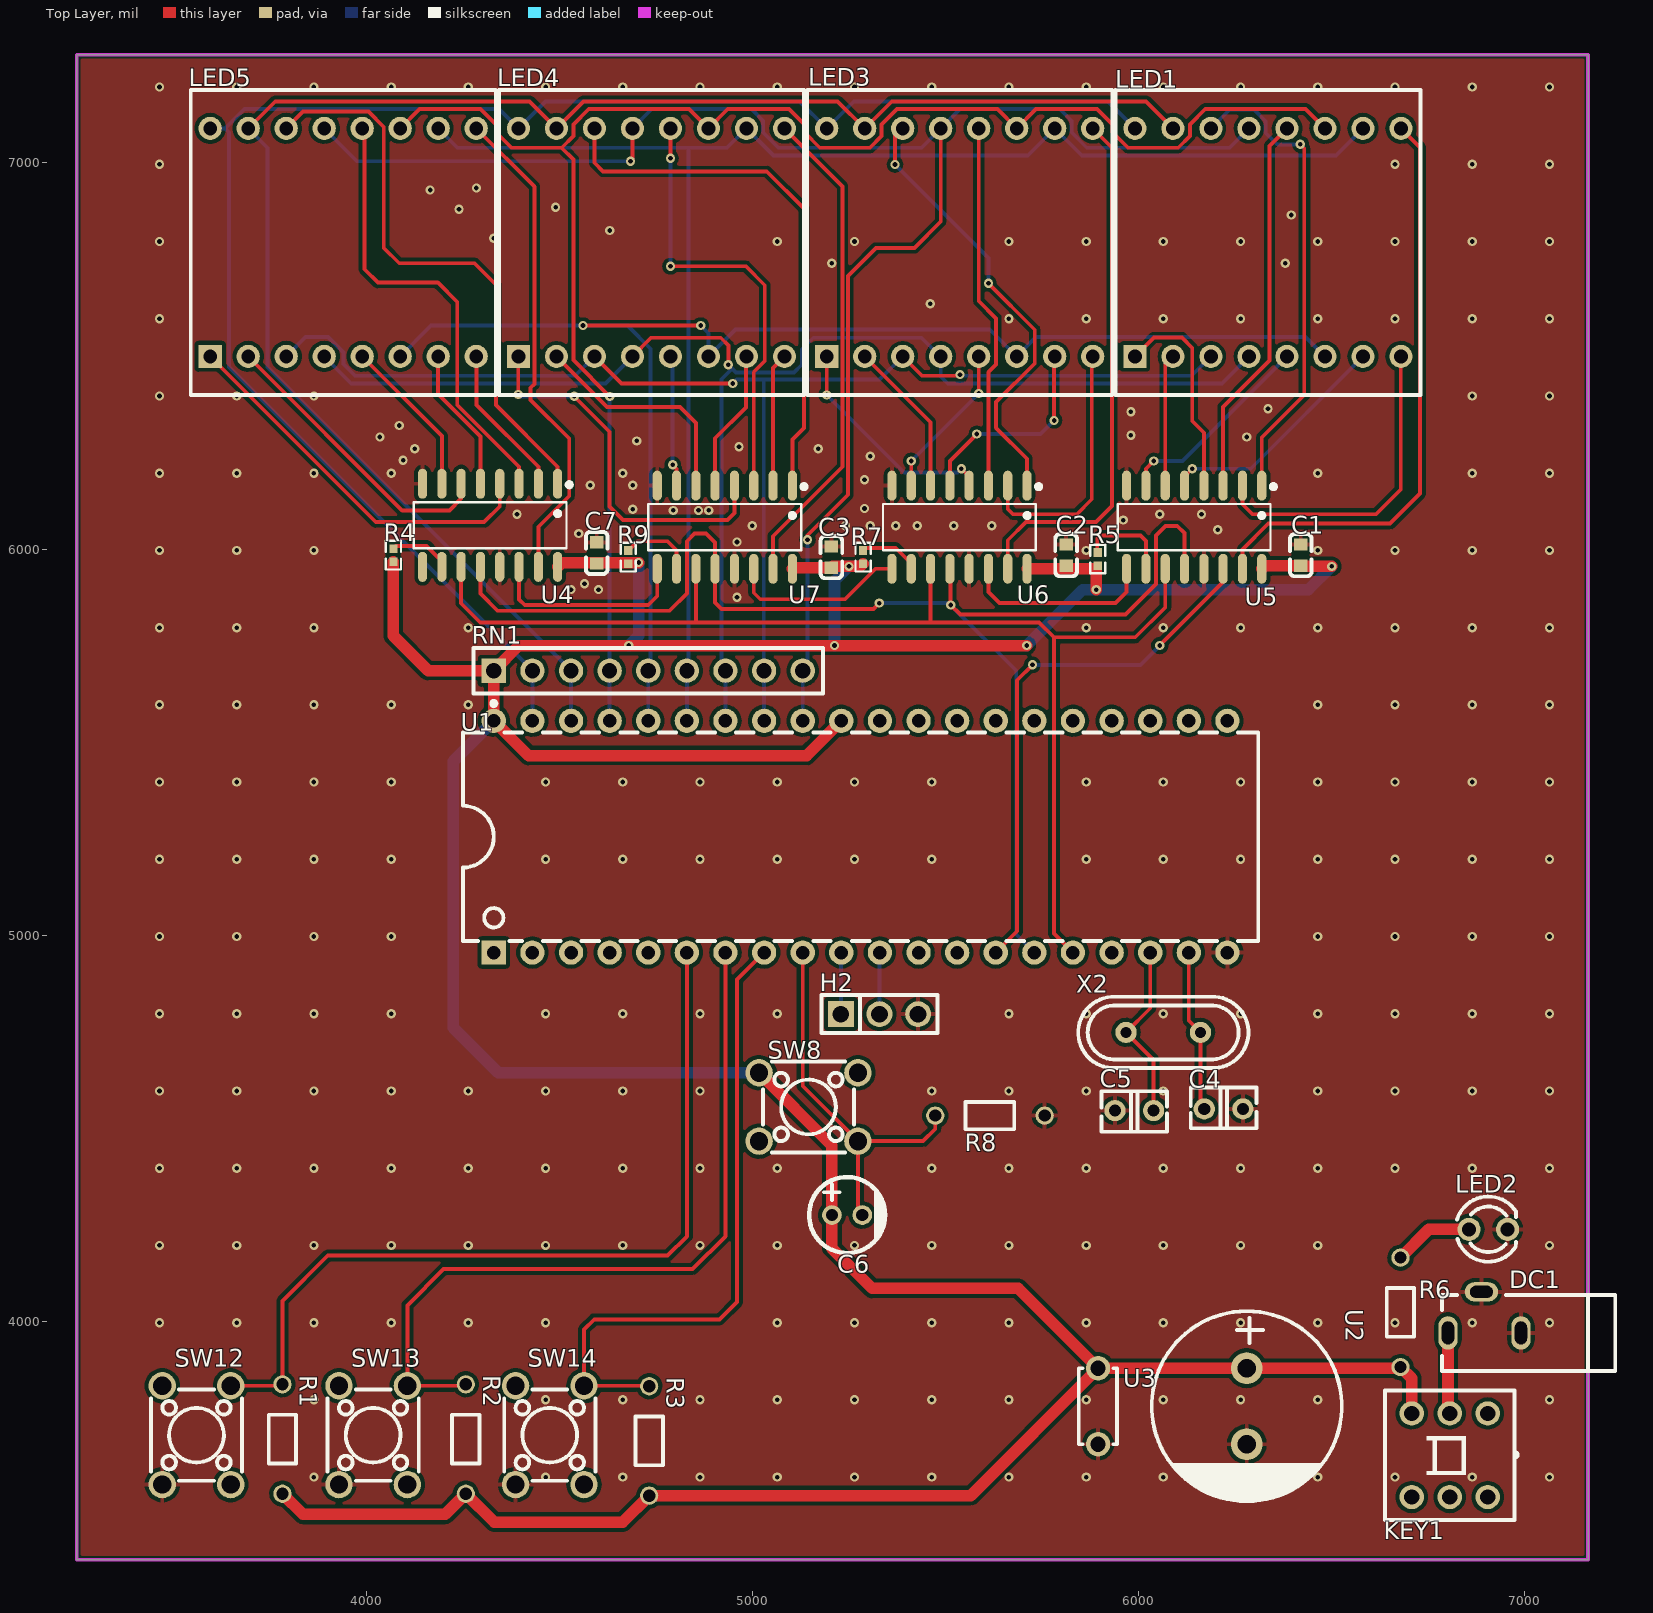
[diagram p0: Top Layer view]
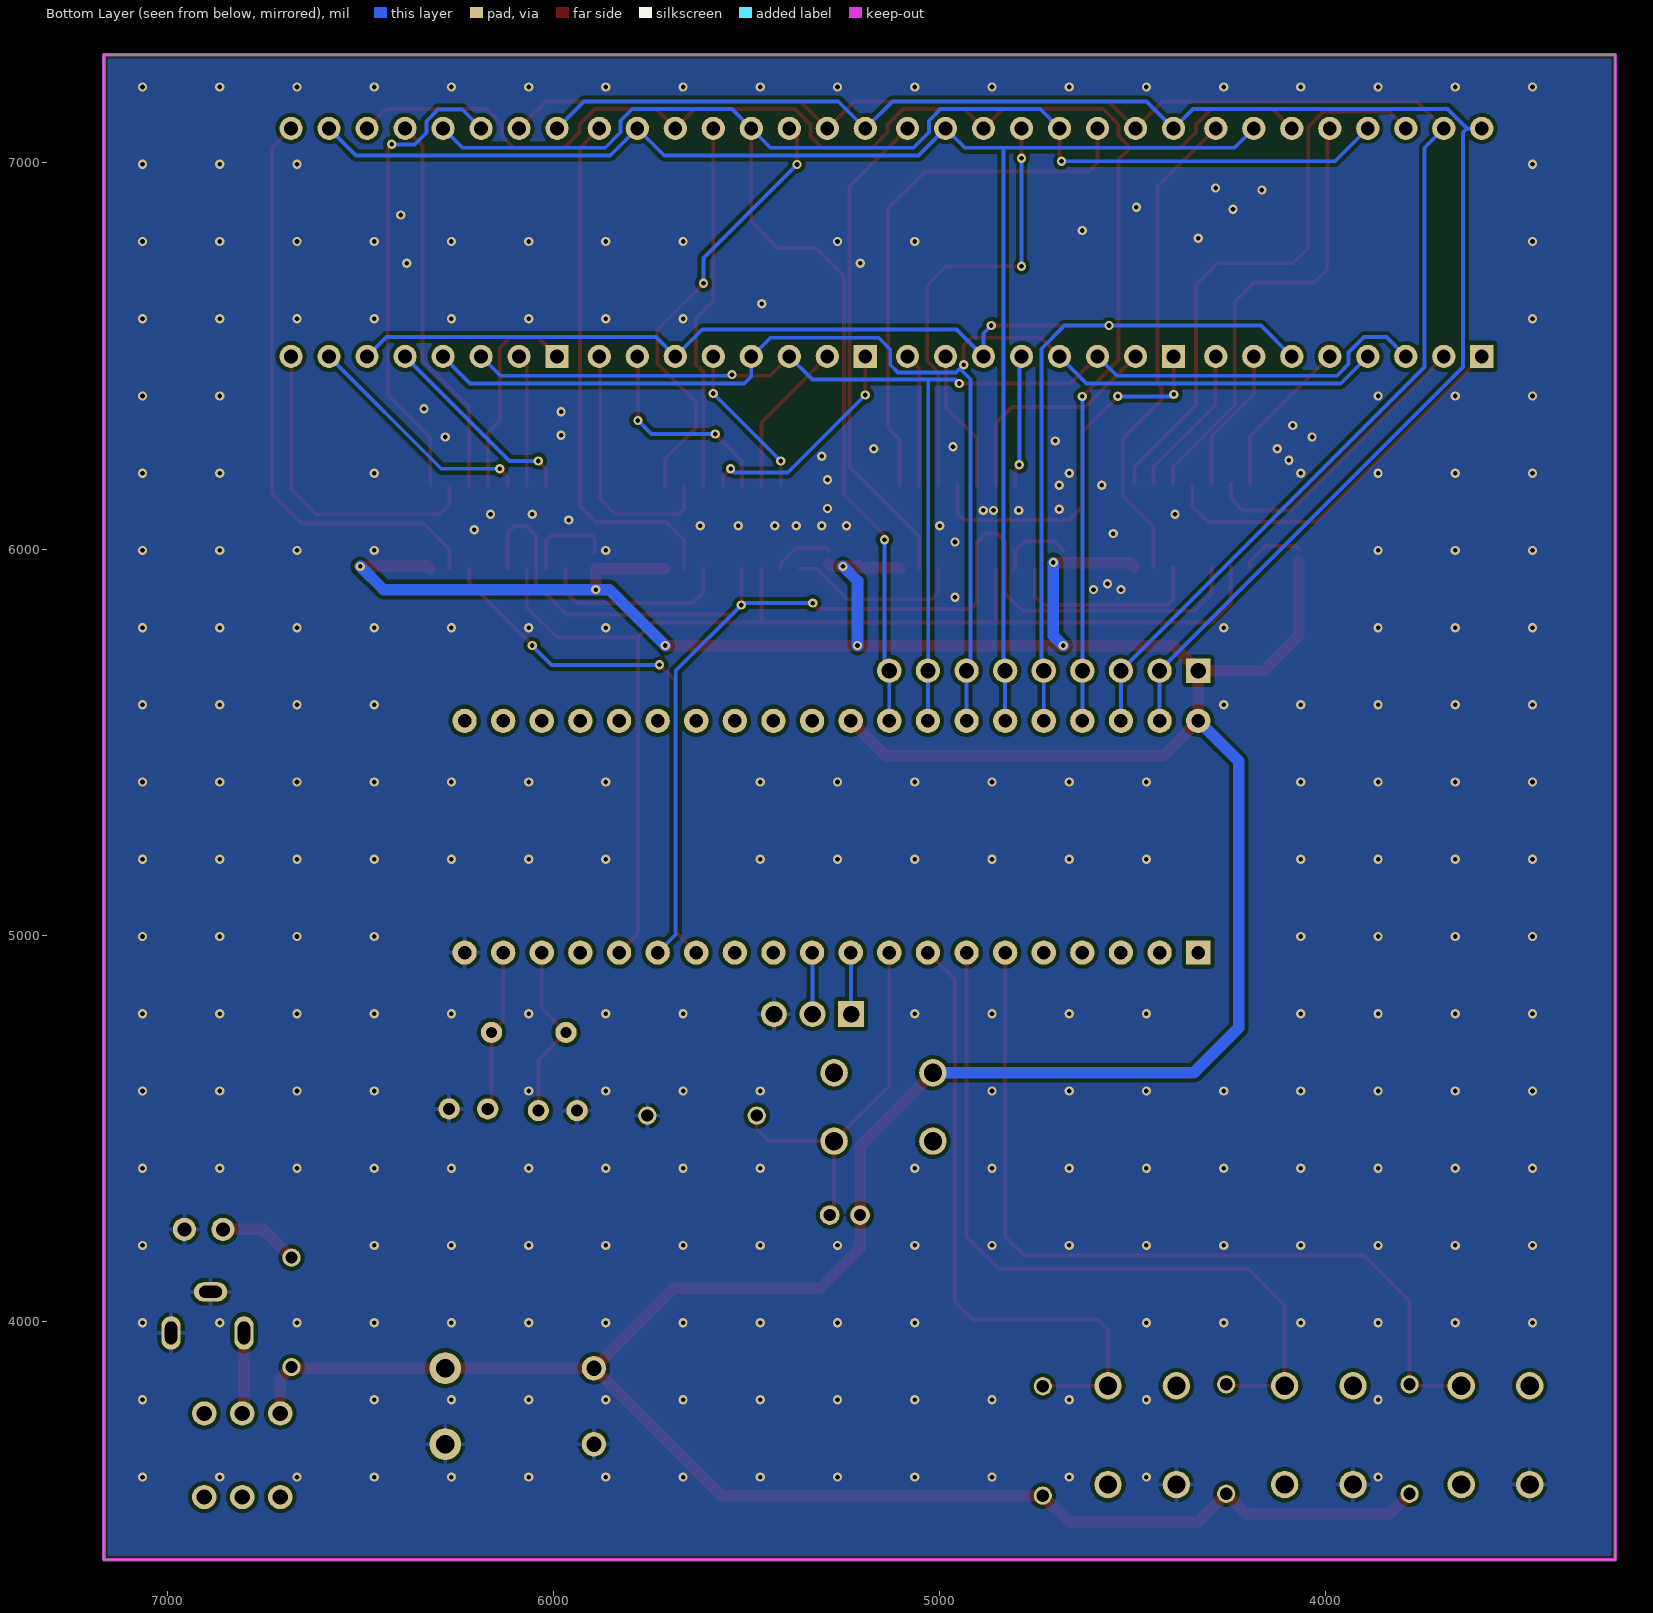
[diagram p1: Bottom Layer view, seen from below]
# Altium PCB MISC62490.pcbdoc
Units mil, origin at the board's own origin, x right, y up, seen from the top; angles counter-clockwise.
Board outline 3914.17 x 3897.64 mil, 2 copper layers (Top Layer, Bottom Layer), stack 62.206 mil thick; 37 components, 78 nets, 245 pads, 321 vias.

## Layer stack, top to bottom
Top Solder Mask Layer: solder mask 0.394, Dk 3.3
Top Layer: signal copper 1.379
Dielectric1: surface 59.449, FR4, Dk 4.5
Bottom Layer: signal copper 1.378
Bottom Solder Mask Layer: solder mask 0.394, Dk 3.3

## Board outline
3250,7280 3250,3382.36 7164.17,3382.36 7164.17,7280

## Design rules (kind name [scope] priority, off if disabled: settings)
BoardOutlineClearance copperThickness2oz_1 [All] p2 off: genericclearance=7.99 ignorepadtopadclearanceinfootprint=FALSE except(0: Arc-SplitContinuation Track-SplitContinuation SMDPad-SplitContinuation THPad-SplitContinuation Via-SplitContinuation Fill-SplitContinuation Region-SplitContinuation Poly-SplitContinuation Text-SplitContinuation Hole-SplitContinuation; 5.98: Arc-CutoutEdge SMDPad-CutoutEdge THPad-CutoutEdge Via-CutoutEdge Fill-CutoutEdge Region-CutoutEdge Text-CutoutEdge; 6.93: Hole-OutlineEdge Hole-CutoutEdge; 10: Poly-OutlineEdge Poly-CutoutEdge; 11.81: Arc-OutlineEdge Track-OutlineEdge SMDPad-OutlineEdge THPad-OutlineEdge Via-OutlineEdge Fill-OutlineEdge Region-OutlineEdge Text-OutlineEdge Track-CutoutEdge)
BoardOutlineClearance copperThickness1oz_1 [All] p4: genericclearance=4.02 ignorepadtopadclearanceinfootprint=FALSE except(0: Arc-SplitContinuation Track-SplitContinuation SMDPad-SplitContinuation THPad-SplitContinuation Via-SplitContinuation Fill-SplitContinuation Region-SplitContinuation Poly-SplitContinuation Text-SplitContinuation Hole-SplitContinuation; 6: SMDPad-CutoutEdge THPad-CutoutEdge Via-CutoutEdge Fill-CutoutEdge Region-CutoutEdge Text-CutoutEdge; 6.93: Hole-OutlineEdge Hole-CutoutEdge; 10: Poly-OutlineEdge Poly-CutoutEdge; 11.8: Arc-OutlineEdge Track-OutlineEdge SMDPad-OutlineEdge THPad-OutlineEdge Via-OutlineEdge Fill-OutlineEdge Region-OutlineEdge Text-OutlineEdge; 11.81: Arc-CutoutEdge Track-CutoutEdge)
Clearance copperThickness2oz [All] p1 off: gap=7.99 ignorepadtopadclearanceinfootprint=FALSE except(5.98: SMDPad-Track SMDPad-SMDPad THPad-Track SMDPad-THPad THPad-THPad Track-Via SMDPad-Via THPad-Via Via-Via Fill-Track Region-Track Fill-SMDPad Region-SMDPad Fill-THPad Region-THPad Fill-Via Region-Via Fill-Fill Fill-Region Region-Region Arc-Track Arc-SMDPad Arc-THPad Arc-Via Fill-Arc Region-Arc Arc-Arc Text-Track SMDPad-Text Text-THPad Text-Via Fill-Text Region-Text Arc-Text Text-Text; 6.93: Hole-Track Hole-SMDPad Hole-THPad Hole-Via Fill-Hole Region-Hole Hole-Arc Hole-Text; 10: Poly-Track Poly-SMDPad Poly-THPad Poly-Via Poly-Fill Poly-Region Poly-Poly Poly-Arc Poly-Text Poly-Hole)
Clearance copperThickness1oz [All] p3: gap=4.02 ignorepadtopadclearanceinfootprint=FALSE except(5.98: SMDPad-Track SMDPad-SMDPad THPad-Track SMDPad-THPad THPad-THPad Track-Via SMDPad-Via THPad-Via Via-Via Fill-Track Region-Track Fill-SMDPad Region-SMDPad Fill-THPad Region-THPad Fill-Via Region-Via Fill-Fill Fill-Region Region-Region; 6: Arc-Track Arc-SMDPad Arc-THPad Arc-Via Fill-Arc Region-Arc Arc-Arc Text-Track SMDPad-Text Text-THPad Text-Via Fill-Text Region-Text Arc-Text Text-Text; 6.93: Hole-Track Hole-SMDPad Hole-THPad Hole-Via Fill-Hole Region-Hole Hole-Arc Hole-Text; 10: Poly-Track Poly-SMDPad Poly-THPad Poly-Via Poly-Fill Poly-Region Poly-Poly Poly-Arc Poly-Text Poly-Hole)
Creepage creepage [All] p1: checkdistance=0 ignoreinternallayers=TRUE applytopolygonpour=TRUE
DiffPairsRouting differentialPair [All] p1: maxlimit=6 minlimit=6 mostfreqgap=6 toplayer_minwidth=5 toplayer_prefwidth=10 toplayer_maxwidth=100 toplayer_mingap=6 toplayer_prefgap=6 toplayer_maxgap=6 bottomlayer_minwidth=5 bottomlayer_prefwidth=10 bottomlayer_maxwidth=100 bottomlayer_mingap=6 bottomlayer_prefgap=6 bottomlayer_maxgap=6 maxuncoupledlength=10
HoleToHoleClearance otherClearance [All] p1: gap=11.81 allowstackedmicrovias=TRUE
Length netLength [All] p1: minlimit=0 maxlimit=0
MatchedLengths netLengthTolerance [All] p1: tolerance=1000
PasteMaskExpansion pasteMaskExpansion [All] p1: expansion=0
PlaneConnect innerPlane [All] p1: planeconnectstyle=Relief reliefexpansion=20 reliefentries=4 reliefconductorwidth=10 reliefairgap=10
PolygonConnect copperRegion [(InNet('GND'))] p1: connectstyle=Relief reliefconductorwidth=10 reliefentries=4 polygonreliefangle="90 Angle" airgapwidth=10 via.connectstyle=Relief via.reliefconductorwidth=10 via.reliefentries=4 via.polygonreliefangle="90 Angle" via.airgapwidth=10
RoutingVias viaSize [All] p1: holewidth=12.01 width=24.02 viastyle="Through Hole" minholewidth=11.81 minwidth=19.68 maxholewidth=248.03 maxwidth=393.7
SolderMaskExpansion solderMaskExpansion [IsVia] p1: expansion=-1000 istentingtop=TRUE
SolderMaskExpansion solderMaskExpansion [All] p2: expansion=2 istentingtop=FALSE
Width copperThickness2oz_2 [All] p1 off: maxlimit=100 minlimit=8 preferedwidth=10
Width copperThickness1oz_2 [All] p2: maxlimit=100 minlimit=5 preferedwidth=10

## Components (designator, comment, footprint, x,y, rotation, side; value= is the part's Value field where it differs from the comment)
C1 "100nF" C0603 6420,5984.05 r270 top
C2 "100nF" C0603 5812.16,5984.05 r270 top
C3 "100nF" C0603 5204.33,5979.05 r270 top
C4 "22pF" CAP-TH_L3.8-W2.5-P2.54-D0.50 6220,4550 r180 top
C5 "22pF" CAP-TH_L3.8-W2.5-P2.54-D0.50 5988.8,4545.73 r0 top
C6 "10uF" CAP-TH_BD5.0-P2.00-D0.8-FD-10UF50VC110GL 5245,4275 r0 top
C7 "100nF" C0603 4596.49,5989.81 r270 top
DC1 "DC-002" DC-IN-TH_DC-3510 6895.71,4023.03 r0 top
H2 "" HDR-TH_3P-P2.54-V-M 5328.8,4795.46 r0 top
KEY1 "Non-latching switch 8.5×8.5 silent" SW-TH_6P-L8.5-W8.5-P2.54 6805.71,3653.03 r180 top
LED1 "SLD0888FR1C1BD-3.5D" LED-MAT-TH_SLD0888FR1C1BD-3.5D 6335,6794.05 r0 top
LED2 "" LED_TH-3mm 6905.71,4238.03 r0 top
LED3 "SLD0888FR1C1BD-3.5D" LED-MAT-TH_SLD0888FR1C1BD-3.5D 5536.66,6794.05 r0 top
LED4 "SLD0888FR1C1BD-3.5D" LED-MAT-TH_SLD0888FR1C1BD-3.5D 4738.33,6794.05 r0 top
LED5 "SLD0888FR1C1BD-3.5D" LED-MAT-TH_SLD0888FR1C1BD-3.5D 3940,6794.05 r0 top
R1 "10kΩ" Res_1/8W 3780,3695 r270 top
R2 "10kΩ" Res_1/8W 4255,3695 r270 top
R3 "10kΩ" Res_1/8W 4730,3690 r270 top
R4 "10kΩ" R0402 4070,5984.05 r270 top
R5 "10kΩ" R0402 5894.07,5974.05 r270 top
R6 "1kΩ" Res_1/8W 6675.71,4023.03 r270 top
R7 "10kΩ" R0402 5286.24,5979.05 r270 top
R8 "10kΩ" Res_1/8W 5615,4535 r180 top
R9 "10kΩ" R0402 4678.4,5979.05 r270 top
RN1 "-" RES-ARRAY-TH_9P-P2.54-D1.0 4730,5685 r0 top
SW8 "" SW-TH_4P-L6.0-W6.0-P4.50-LS6.5 5145,4555 r0 top
SW12 "" SW-TH_4P-L6.0-W6.0-P4.50-LS6.5 3560,3705 r270 top
SW13 "" SW-TH_4P-L6.0-W6.0-P4.50-LS6.5 4017.5,3705 r270 top
SW14 "" SW-TH_4P-L6.0-W6.0-P4.50-LS6.5 4475,3705 r270 top
U1 "STC89C52RC-40I-PDIP40" DIP-40_L52.0-W13.7-P2.54-LS15.2-BL 5280,5255 r0 top
U2 "1000uF" CAP-TH_BD12.5-P5.00-D0.6-FD 6280,3780 r270 top
U3 "100nF" CAP-TH_L5.0-W2.5-P5.00-D1.0 5895,3780 r270 top
U4 "74HC595D,118" SOIC-16_L9.9-W3.9-P1.27-LS6.0-BL 4320.4,6061.5 r180 top
U5 "74HC595D,118" SOIC-16_L9.9-W3.9-P1.27-LS6.0-BL 6143.9,6056.5 r180 top
U6 "74HC595D,118" SOIC-16_L9.9-W3.9-P1.27-LS6.0-BL 5536.07,6056.5 r180 top
U7 "74HC595D,118" SOIC-16_L9.9-W3.9-P1.27-LS6.0-BL 4928.23,6056.5 r180 top
X2 "11.0592MHz" OSC-TH_L11.1-W4.7-P4.88 6063.8,4748.02 r0 top

## Footprints (in the part's own frame and the unit in brackets; to place one, negate y for a bottom-side part, rotate by r counter-clockwise, add the part's x,y. Pads: shape width x height; smd on the part's side, far side on the other; paste and mask are expansions set on the pad)
C0603 [mm]
  rect 0.8x0.9 smd: 1(-0.7,0) 2(0.7,0)
  silkscreen extent -1.39,-0.71 1.39,0.71
CAP-TH_BD5.0-P2.00-D0.8-FD-10UF50VC110GL [mm]
  round 1.3 hole 0.8: 1(-1,0) 2(1,0)
  silkscreen extent -2.5,-2.5 2.5,2.5
CAP-TH_BD12.5-P5.00-D0.6-FD [mm]
  round 2.1 hole 1.2 paste+0 mask+0.05: 1(-2.5,0) 2(2.5,0)
  silkscreen extent -6.25,-6.25 6.25,6.25
CAP-TH_L3.8-W2.5-P2.54-D0.50 [mm]
  round 1.4 hole 0.8 paste+0 mask+0.05: 1(-1.27,0) 2(1.27,0)
  silkscreen extent -2.16,-1.4 2.16,1.27
CAP-TH_L5.0-W2.5-P5.00-D1.0 [mm]
  round 1.6 hole 1: 1(-2.5,0) 2(2.5,0)
  silkscreen extent -2.5,-1.27 2.5,1.25
DC-IN-TH_DC-3510 [mm]
  oval 1.27x2.2 hole 0.8 slot 1.5 at 90 deg: 1(-2.4,-1.35) 2(2.4,-1.35)
  oval 2.2x1.27 hole 0.8 slot 1.5 at 0 deg: 3(-0.2,1.35)
  silkscreen extent -2.8,-3.85 8.6,1.15
DIP-40_L52.0-W13.7-P2.54-LS15.2-BL [mil]
  rect 63x63 hole 35: 1(-950,-300)
  round 63 hole 35: 2(-850,-300) 3(-750,-300) 4(-650,-300) 5(-550,-300) 6(-450,-300) 7(-350,-300) 8(-250,-300) 9(-150,-300) 10(-50,-300) 11(50,-300) 12(150,-300) 13(250,-300) 14(350,-300) 15(450,-300) 16(550,-300) 17(650,-300) 18(750,-300) 19(850,-300) 20(950,-300) 21(950,300) 22(850,300) 23(750,300) 24(650,300) 25(550,300) 26(450,300) 27(350,300) 28(250,300) 29(150,300) 30(50,300) 31(-50,300) 32(-150,300) 33(-250,300) 34(-350,300) 35(-450,300) 36(-550,300) 37(-650,300) 38(-750,300) 39(-850,300) 40(-950,300)
  silkscreen extent -1030,-270 1030,270
HDR-TH_3P-P2.54-V-M [mm]
  rect 1.7x1.7 hole 1.1: 1(-2.54,0)
  round 1.7 hole 1.1: 2(0,0) 3(2.54,0)
  silkscreen extent -3.81,-1.25 3.81,1.25
LED-MAT-TH_SLD0888FR1C1BD-3.5D [mil]
  rect 60x60 hole 36: 1(-344.49,-295.28)
  round 60 hole 36: 2(-246.06,-295.28) 3(-147.64,-295.28) 4(-49.21,-295.28) 5(49.21,-295.28) 6(147.64,-295.28) 7(246.06,-295.28) 8(344.49,-295.28) 9(344.49,295.27) 10(246.06,295.27) 11(147.64,295.27) 12(49.21,295.27) 13(-49.21,295.27) 14(-147.64,295.27) 15(-246.06,295.27) 16(-344.49,295.27)
  silkscreen extent -395,-395 395,395
LED_TH-3mm [mil]
  round 60 hole 36 paste+0 mask+2: 1(-50,0) 2(50,0)
  silkscreen extent -81,-84 72,85
OSC-TH_L11.1-W4.7-P4.88 [mm]
  round 1.4 hole 0.7: 1(-2.45,0) 2(2.45,0)
  silkscreen extent -5.59,-2.35 5.6,2.35
R0402 [mm]
  rect 0.566x0.54 smd paste-100 mask+0.051: 1(-0.433,0) 2(0.433,0)
  silkscreen extent -0.94,-0.5 0.94,0.5
RES-ARRAY-TH_9P-P2.54-D1.0 [mm]
  rect 1.6x1.6 hole 1: 1(-10.16,0)
  round 1.6 hole 1: 2(-7.62,0) 3(-5.08,0) 4(-2.54,0) 5(0,0) 6(2.54,0) 7(5.08,0) 8(7.62,0) 9(10.16,0)
  silkscreen extent -11.5,-2.31 11.5,1.5
Res_1/8W [mil]
  round 47.2 hole 31.5 paste+0 mask+2: 1(-141.7,2.48) 2(141.7,2.48)
  silkscreen extent -63,-33 63,38
SOIC-16_L9.9-W3.9-P1.27-LS6.0-BL [mil]
  oval 23.7x77.6 smd: 1(-175,-107.7) 2(-125,-107.7) 3(-75,-107.7) 4(-25,-107.7) 5(25,-107.7) 6(75,-107.7) 7(125,-107.7) 8(175,-107.7) 9(175,107.7) 10(125,107.7) 11(75,107.7) 12(25,107.7) 13(-25,107.7) 14(-75,107.7) 15(-125,107.7) 16(-175,107.7)
  silkscreen extent -211,-111 198,60
SW-TH_4P-L6.0-W6.0-P4.50-LS6.5 [mm]
  round 1.8 hole 1.2: 1(-3.25,2.25) 2(3.25,2.25) 3(-3.25,-2.25) 4(3.25,-2.25)
  silkscreen extent -3,-3 3,3
SW-TH_6P-L8.5-W8.5-P2.54 [mm]
  round 1.6 hole 1: 1(-2.5,-2.75) 2(0,-2.75) 3(2.5,-2.75) 4(-2.5,2.75) 5(0,2.75) 6(2.5,2.75)
  silkscreen extent -4.47,-4.25 4.25,4.25

## Via types
v1: diameter 24.02, hole 12, Top Layer to Bottom Layer, 321 vias

## Nets (pads, with @x,y where several pads share a name; then routed paths per layer and width w, separated by ;. In a path a pad name is that pad's centre, name@x,y a point inside that pad or via, vN(x,y) a via of type N, cw(c..) or ccw(c..) an arc to the next point about the centre after c; other vN are vias at no path point)
$1N111: LED2.1 R6.1 | length 207.9
  Top Layer w30: R6.1 6751.49,4238.03 LED2.1
$1N113: DC1.1 KEY1.2 | length 210.4
  Top Layer w30: DC1.1 6801.22,3765.8 KEY1.2
$1N208: R4.1 U4.10 | length 158.5
  Top Layer w10: R4.1 4076.5,6007.6 4155.4,6007.6 4195.4,5967.6 U4.10
$1N209: R9.1 U7.10 | length 192.3
  Top Layer w10: R9.1 4702.31,6020 4780,6020 4803.24,5996.76 U7.10
$1N210: R7.1 U6.10 | length 157.9
  Top Layer w10: R7.1 5292.74,6002.6 5371.07,6002.6 5411.07,5962.6 U6.10
$1N211: R5.1 U5.10 | length 244.3
  Top Layer w10: R5.1 5892.93,5992.23 5892.93,6027.93 5900,6035 6005,6035 6018.9,6021.1 U5.10
$1N212: U4.14 U7.9 | length 528.3
  Top Layer w10: U4.14 4395.4,5869.6 4410,5855 4730,5855 4753.24,5878.24 U7.9
$1N213: U6.9 U7.14 | length 459.5
  Top Layer w10: U7.14 5003.23,5886.77 5020,5870 5240,5870 5318.8,5948.8 U6.9
$1N214: U5.9 U6.14 | length 501.6
  Top Layer w10: U6.14 5611.07,5888.93 5640,5860 5940,5860 5968.9,5888.9 U5.9
A0: LED1.9 U5.15 | length 1536.1
  Top Layer w10: U5.15 6268.91,5998.91 6335.73,6065.73 6650.73,6065.73 6728.9,6143.9 6728.9,7039.91 LED1.9
A1: LED1.14 U5.1 | length 1240.1
  Top Layer w10: U5.1 6318.91,6288.91 6428.91,6398.91 6428.91,7038 v1(6418.91,7048)
  Bottom Layer w10: LED1.14 6236.03,7138 6298.91,7138 6328.91,7108 6328.91,7078 6358.91,7048 v1(6418.91,7048)
A2: LED1.8 U5.2 | length 840.5
  Top Layer w10: U5.2 6268.91,6116.09 6295,6090 6615,6090 6678.9,6153.9 6678.9,6498.2 LED1.8
A3: LED1.12 U5.3 | length 993.6
  Top Layer w10: U5.3 6218.91,6368 6338.91,6488 6338.91,7044.03 LED1.12
A4: LED1.1 U5.4 | length 549.2
  Top Layer w10: LED1.1 6039.73,6548 6112,6548 6138.91,6521.09 6138.91,6331.09 6168.91,6301.09 U5.4
A5: LED1.7 U5.5 | length 614.7
  Top Layer w10: U5.5 6118.91,6188 v1(6138.91,6208)
  Bottom Layer w10: v1(6138.91,6208) 6290.28,6208 LED1.7
A6: LED1.2 U5.6 | length 342.9
  Top Layer w10: U5.6 6068.91,6478.75 LED1.2
A7: LED1.5 U5.7 | length 529.5
  Top Layer w10: U5.7 6018.91,6208 v1(6038.91,6228)
  Bottom Layer w10: v1(6038.91,6228) 6113.43,6228 LED1.5
A8: LED3.9 U6.15 | length 1379.4
  Top Layer w10: U6.15 5661.07,6022.6 5708.47,6070 5890,6070 5931.07,6111.07 5931.07,7039.42 LED3.9@5881.15,7089.33
A9: LED3.14 U6.1 | length 1157.9
  Top Layer w10: v1(5369.03,6995.96) 5369.03,7069.33 LED3.14 ; v1(5611.07,6688) 5731.07,6568 5731.07,6480.84 5631.07,6380.84 5631.07,6313.93 5711.07,6233.93 U6.1
  Bottom Layer w10: v1(5369.03,6995.96) 5611.07,6753.92 v1(5611.07,6688)
A10: LED3.8 U6.2 | length 670.8
  Top Layer w10: U6.2 5661.07,6103.93 5675,6090 5840,6090 5878.77,6128.77 5878.77,6496.39 LED3.8@5881.15,6498.78
A11: LED3.12 U6.3 | length 952.1
  Top Layer w10: LED3.12 5585.88,6641.94 5631.07,6596.74 5631.07,6478 5611.07,6458 U6.3
A12: LED3.1 U6.4 | length 588.3
  Top Layer w10: v1(5192.18,6398.78) LED3.1 ; v1(5541.07,6208) 5561.07,6188 U6.4
  Bottom Layer w10: v1(5192.18,6398.78) 5392.95,6198 5531.07,6198 v1(5541.07,6208)
A13: LED3.7 U6.5 | length 543.8
  Top Layer w10: U6.5 5511.07,6228 v1(5581.07,6298) ; v1(5781.07,6333) 5781.07,6497.12 LED3.7
  Bottom Layer w10: v1(5581.07,6298) 5746.07,6298 v1(5781.07,6333)
A14: LED3.2 U6.6 | length 405.2
  Top Layer w10: LED3.2 5461.07,6328.31 U6.6
A15: LED3.5 U6.7 | length 407
  Top Layer w10: U6.7 v1(5411.07,6228) ; v1(5585.88,6402.81) LED3.5
  Bottom Layer w10: v1(5411.07,6228) v1(5585.88,6402.81)
A16: LED4.9 U7.15 | length 1277.4
  Top Layer w10: U7.15 5053.23,6033.23 5233.23,6213.23 5233.23,6938.92 LED4.9
A17: LED4.14 U7.1 | length 1410.5
  Top Layer w10: LED4.14 4590.69,7000.55 4613.24,6978 5037,6978 5133.23,6881.77 5133.23,6313.23 5103.23,6283.23 U7.1
A18: LED4.8 U7.2 | length 346.8
  Top Layer w10: U7.2 5053.23,6469.19 LED4.8
A19: LED4.12 U7.3 | length 1152.5
  Top Layer w10: v1(4787.54,6732.31) 4982.69,6732.31 5031.85,6683.15 5031.85,6486.62 5003.23,6458 U7.3 ; v1(4787.54,7012.31) LED4.12
  Bottom Layer w10: v1(4787.54,6732.31) v1(4787.54,7012.31)
A20: LED4.1 U7.4 | length 985.4
  Top Layer w10: v1(4393.24,6400.41) 4393.24,6498.17 LED4.1 ; v1(4538.24,6395.41) 4630,6303.64 4630,6110 4665,6075 4935,6075 4953.23,6093.23 U7.4
  Bottom Layer w10: v1(4393.24,6400.41) 4398.24,6395.41 v1(4538.24,6395.41)
A21: LED4.7 U7.5 | length 368.2
  Top Layer w10: U7.5 4903.23,6286.74 4983.23,6366.74 4983.23,6497.62 LED4.7
A22: LED4.2 U7.6 | length 594.8
  Top Layer w10: LED4.2 4623.05,6368 4812,6368 4853.23,6326.77 U7.6
A23: LED4.5 U7.7 | length 341.1
  Top Layer w10: v1(4793.24,6218) 4803.24,6208 U7.7
  Bottom Layer w10: LED4.5 4793.24,6493.09 v1(4793.24,6218)
A24: LED5.9 U4.15 | length 1276.7
  Top Layer w10: LED5.9 4435.4,6938.42 4435.4,6427.6 4425.4,6417.6 4425.4,6386.34 4525.4,6286.34 4525.4,6137.6 4445.4,6057.6 U4.15
A25: LED5.14 U4.1 | length 1512.1
  Top Layer w10: LED5.14 3836.03,7133 4005.4,7133 4045,7093.4 4045,6780 4085,6740 4280,6740 4335.4,6684.6 4335.4,6373 4495.4,6213 U4.1
A26: LED5.8 U4.2 | length 396.2
  Top Layer w10: LED5.8 4285.4,6497.87 4285.4,6373 4445.4,6213 U4.2
A27: LED5.12 U4.3 | length 1179.2
  Top Layer w10: LED5.12 3995.4,7083.14 3995.4,6724.6 4030,6690 4185,6690 4235.4,6639.6 4235.4,6373 4395.4,6213 U4.3
A28: LED5.1 U4.4 | length 1003
  Top Layer w10: LED5.1 4024.29,6070 4305,6070 4345.4,6110.4 U4.4
A29: LED5.7 U4.5 | length 375.4
  Top Layer w10: LED5.7 4185.4,6498.12 4185.4,6401.74 4295.4,6291.74 U4.5
A30: LED5.2 U4.6 | length 768
  Top Layer w10: LED5.2 4092.72,6100 4215,6100 4245.4,6130.4 U4.6
A31: LED5.5 U4.7 | length 415
  Top Layer w10: LED5.5 4195.4,6292.59 U4.7
CLK: U1.16 U4.11 U5.11 U6.11 U7.11 | length 3201.4
  Top Layer w10: U4.11 4245.4,5859.6 4295,5810 4853.23,5810 ; U7.11 4853.23,5810.01 ; U6.11 5461.07,5812.07 5459,5810 ; U1.16 5781.07,5003.94 5781.07,5771.4 ; U5.11 6068.9,5848.9 5991.4,5771.4 5781.07,5771.4 ; 4853.23,5810 5459,5810 ; 5459,5810 5742.47,5810 5781.07,5771.4
DI: U1.14 U5.14 | length 1401.4
  Top Layer w10: U1.14 5685,5010 5685,5660 v1(5725,5700) ; v1@6054.45,5750.55 6218.91,5915 U5.14
  Bottom Layer w10: v1(5725,5700) 6005,5700 v1(6055,5750)
GND: C1.1 C2.1 C3.1 C4.1 C5.1 C7.1 DC1.2 DC1.3 H2.3 LED2.2 R8.1 SW12.4 SW13.4 SW14.4 U1.20 U2.2 U3.2 U4.8 U4.13 U5.8 U5.13 U6.8 U6.13 U7.8 U7.13
  other v1: 3864.1,3596.46 4464.1,3596.46 4664.1,3596.46 4864.1,3596.46 5064.1,3596.46 5264.1,3596.46 5464.1,3596.46 5664.1,3596.46 5864.1,3596.46 6064.1,3596.46 6264.1,3596.46 6464.1,3596.46 6664.1,3596.46 6864.1,3596.46 7064.1,3596.46 3864.1,3796.46 4464.1,3796.46 4664.1,3796.46 4864.1,3796.46 5064.1,3796.46 5264.1,3796.46 5464.1,3796.46 5664.1,3796.46 5864.1,3796.46 6064.1,3796.46 6264.1,3796.46 6464.1,3796.46 7064.1,3796.46 3464.1,3996.46 3664.1,3996.46 3864.1,3996.46 4064.1,3996.46 4264.1,3996.46 4464.1,3996.46 5064.1,3996.46 5264.1,3996.46 5464.1,3996.46 5664.1,3996.46 5864.1,3996.46 6064.1,3996.46 6264.1,3996.46 6464.1,3996.46 6664.1,3996.46 6864.1,3996.46 7064.1,3996.46 3464.1,4196.46 3664.1,4196.46 3864.1,4196.46 4064.1,4196.46 4264.1,4196.46 4464.1,4196.46 4664.1,4196.46 4864.1,4196.46 5064.1,4196.46 5264.1,4196.46 5464.1,4196.46 5664.1,4196.46 5864.1,4196.46 6064.1,4196.46 6264.1,4196.46 6464.1,4196.46 7064.1,4196.46 3464.1,4396.46 3664.1,4396.46 3864.1,4396.46 4064.1,4396.46 4264.1,4396.46 4464.1,4396.46 4664.1,4396.46 4864.1,4396.46 5064.1,4396.46 5464.1,4396.46 5664.1,4396.46 5864.1,4396.46 6064.1,4396.46 6264.1,4396.46 6464.1,4396.46 6664.1,4396.46 6864.1,4396.46 7064.1,4396.46 3464.1,4596.46 3664.1,4596.46 3864.1,4596.46 4064.1,4596.46 4264.1,4596.46 4464.1,4596.46 4664.1,4596.46 4864.1,4596.46 5464.1,4596.46 5664.1,4596.46 5864.1,4596.46 6064.1,4596.46 6464.1,4596.46 6664.1,4596.46 6864.1,4596.46 7064.1,4596.46 3464.1,4796.46 3664.1,4796.46 3864.1,4796.46 4064.1,4796.46 4464.1,4796.46 4664.1,4796.46 4864.1,4796.46 5064.1,4796.46 5664.1,4796.46 5864.1,4796.46 6064.1,4796.46 6264.1,4796.46 6464.1,4796.46 6664.1,4796.46 6864.1,4796.46 7064.1,4796.46 3464.1,4996.46 3664.1,4996.46 3864.1,4996.46 4064.1,4996.46 6464.1,4996.46 6664.1,4996.46 6864.1,4996.46 7064.1,4996.46 3464.1,5196.46 3664.1,5196.46 3864.1,5196.46 4064.1,5196.46 4464.1,5196.46 4664.1,5196.46 4864.1,5196.46 5064.1,5196.46 5264.1,5196.46 5464.1,5196.46 5864.1,5196.46 6064.1,5196.46 6264.1,5196.46 6464.1,5196.46 6664.1,5196.46 6864.1,5196.46 7064.1,5196.46 3464.1,5396.46 3664.1,5396.46 3864.1,5396.46 4064.1,5396.46 4464.1,5396.46 4664.1,5396.46 4864.1,5396.46 5064.1,5396.46 5264.1,5396.46 5464.1,5396.46 5864.1,5396.46 6064.1,5396.46 6264.1,5396.46 6464.1,5396.46 6664.1,5396.46 6864.1,5396.46 7064.1,5396.46 3464.1,5596.46 3664.1,5596.46 3864.1,5596.46 4064.1,5596.46 4264.1,5596.46 6464.1,5596.46 6664.1,5596.46 6864.1,5596.46 7064.1,5596.46 3464.1,5796.46 3664.1,5796.46 3864.1,5796.46 4264.1,5796.46 5864.1,5796.46 6064.1,5796.46 6264.1,5796.46 6464.1,5796.46 6664.1,5796.46 6864.1,5796.46 7064.1,5796.46 4960,5875 4530,5895 4601.13,5895 4565,5910 3464.1,5996.46 3664.1,5996.46 3864.1,5996.46 5864.1,5996.46 6464.1,5996.46 6664.1,5996.46 6864.1,5996.46 7064.1,5996.46 4960,6018.11 4550,6040 6205,6050 4999.51,6060.03 5240.86,6060.03 5304.89,6060.03 5370.84,6060.03 5426.42,6060.03 5521.42,6060.03 5619.93,6060.03 5960,6075 4390,6090 6055,6090 6162.68,6090 4795,6100 4860,6100 4887,6100 4690,6102.69 5290,6105 4580,6165 4690,6165 5290,6179.24 3464.1,6196.46 3664.1,6196.46 3864.1,6196.46 4064.1,6196.46 4664.1,6196.46 6464.1,6196.46 6864.1,6196.46 7064.1,6196.46 4095,6230 5305,6240 4125,6260 5170,6260 4965,6265 4700,6280 4035,6290 6280,6290 5980,6295 4085,6320 5980,6355.3 6335,6363.37 3464.1,6396.46 3664.1,6396.46 3864.1,6396.46 6864.1,6396.46 7064.1,6396.46 3464.1,6596.46 5664.1,6596.46 5864.1,6596.46 6064.1,6596.46 6264.1,6596.46 6464.1,6596.46 6664.1,6596.46 6864.1,6596.46 7064.1,6596.46 5460,6635 5205,6740 6380,6740 3464.1,6796.46 5064.1,6796.46 5264.1,6796.46 5664.1,6796.46 5864.1,6796.46 6064.1,6796.46 6264.1,6796.46 6464.1,6796.46 6664.1,6796.46 6864.1,6796.46 7064.1,6796.46 4330,6805 4630,6825 6395,6865 4240,6880 4490,6885 4165,6930 4285,6935 3464.1,6996.46 6664.1,6996.46 6864.1,6996.46 7064.1,6996.46 3464.1,7196.46 3664.1,7196.46 3864.1,7196.46 4064.1,7196.46 4264.1,7196.46 4464.1,7196.46 4664.1,7196.46 4864.1,7196.46 5064.1,7196.46 5264.1,7196.46 5464.1,7196.46 5664.1,7196.46 5864.1,7196.46 6064.1,7196.46 6264.1,7196.46 6464.1,7196.46 6664.1,7196.46 6864.1,7196.46 7064.1,7196.46
P00: LED1.16 LED3.16 LED4.16 LED5.16 RN1.2 U1.39 | length 4416.5
  Bottom Layer w10: LED5.16 3633.84,7089.33 ; U1.39 RN1.2 3643.84,6471.16 3643.84,7079.33 3633.84,7089.33 ; LED1.16 5920.51,7159.33 5262.18,7159.33 LED3.16 5122.18,7159.33 4463.84,7159.33 LED4.16 4343.84,7139.33 3683.84,7139.33 3633.84,7089.33
P01: LED1.15 LED3.15 LED4.15 LED5.15 RN1.3 U1.38 | length 4449.6
  Top Layer w10: LED5.15 3763.94,7159.33 4422.27,7159.33 LED4.15 4562.27,7159.33 5220.6,7159.33 LED3.15 5360.6,7159.33 6018.94,7159.33 LED1.15
  Bottom Layer w10: LED5.15 3743.94,7039.33 3743.94,6471.06 RN1.3 U1.38
P02: LED1.11 LED3.11 LED4.11 LED5.11 RN1.4 U1.37 | length 4391.5
  Top Layer w10: LED5.11 4137.64,7139.33 4295.97,7139.33 4335.97,7099.33 4335.97,7079.33 4375.97,7039.33 4505.67,7039.33 ; v1(4630,6395.3) 4535.97,6489.33 4535.97,7009.03 4505.67,7039.33 ; LED1.11 6432.64,7139.33 6172.64,7139.33 6132.64,7099.33 6132.64,7069.33 6102.64,7039.33 5972.64,7039.33 5932.64,7079.33 5932.64,7099.33 5892.64,7139.33 5734.3,7139.33 LED3.11 5634.3,7139.33 5374.3,7139.33 5334.3,7099.33 5334.3,7069.33 5304.31,7039.33 5174.31,7039.33 5134.31,7079.33 5134.31,7099.33 5094.31,7139.33 4935.97,7139.33 LED4.11 4835.97,7139.33 4575.97,7139.33 4535.97,7099.33 4535.97,7069.33 4505.97,7039.33 4505.67,7039.33
  Bottom Layer w10: U1.37 RN1.4 v1(4630,6395.3)
P03: LED1.6 LED3.6 LED4.6 LED5.6 RN1.5 U1.36 | length 3761.9
  Top Layer w10: v1(4560.97,6578.78) v1(4865.97,6578.78)
  Bottom Layer w10: LED5.6 4167.64,6578.78 v1(4560.97,6578.78) 4675.97,6578.78 4735.97,6518.78 4735.97,5690.97 RN1.5 U1.36 ; v1(4865.97,6578.78) 4885.97,6558.78 LED4.6 4955.97,6568.78 5614.3,6568.78 LED3.6 5734.3,6548.78 6432.64,6548.78 LED1.6
P04: LED1.10 LED3.10 LED4.10 LED5.10 RN1.6 U1.35 | length 4038.5
  Bottom Layer w10: LED5.10 4236.06,7039.33 4834.39,7039.33 ; U1.35 RN1.6 4834.39,5689.39 4834.39,7039.33 ; LED1.10 6511.06,7019.33 5852.73,7019.33 LED3.10 5712.73,7019.33 5054.39,7019.33 LED4.10 4934.39,7039.33 4834.39,7039.33
P05: LED1.4 LED3.4 LED4.4 LED5.4 RN1.7 U1.34 | length 3637.1
  Top Layer w10: LED4.4 4737.46,6547.11 4917.89,6547.11 4937.46,6527.54 v1(4937.46,6477.11)
  Bottom Layer w10: LED5.4 3960.79,6428.78 4619.12,6428.78 LED4.4 ; U1.34 RN1.7 4920,5695 4920,6439.66 4947.46,6467.11 ; v1(4937.46,6477.11) 4957.46,6457.11 5107.45,6457.11 5127.45,6477.11 5127.45,6517.11 5157.45,6547.11 5437.45,6547.11 LED3.4@5487.45,6497.11 ; LED3.4@5487.45,6498.78 5487.45,6447.11 5505.79,6428.78 6215.79,6428.78 LED1.4
P06: LED1.3 LED3.3 LED4.3 LED5.3 RN1.8 U1.33 | length 3481.5
  Top Layer w10: LED4.3 4660.69,6428.78 v1(4949.03,6428.78) ; LED3.3 5439.03,6448.78 5534.37,6448.78 v1(5537.36,6451.77)
  Bottom Layer w10: LED5.3 3842.36,6548.78 3900.69,6548.78 3940.69,6508.78 3940.69,6478.78 3970.69,6448.78 4540.69,6448.78 LED4.3 ; v1(4949.03,6428.78) 4959.03,6438.78 5329.03,6438.78 LED3.3 ; 5029.03,6438.78 5029.03,5685.97 RN1.8 U1.33 ; v1(5537.36,6451.77) 5540.35,6448.78 6137.36,6448.78 LED1.3
P07: LED1.13 LED3.13 LED4.13 LED5.13 RN1.9 U1.32 | length 4453.8
  Top Layer w10: v1(4684.12,7004.33) 4689.12,7009.33 LED4.13 ; v1(5142.45,6024.33) 5142.45,6035.59 5247.45,6140.59 5247.45,6707.45 5320,6780 5419.45,6780 5487.45,6848.01 LED3.13@5487.45,7089.33
  Bottom Layer w10: LED5.13 3975.79,7004.33 v1(4684.12,7004.33) ; LED4.13 4739.12,7139.33 4997.46,7139.33 5027.46,7109.33 5027.46,7079.33 5067.46,7039.33 5437.45,7039.33 5487.45,7089.33 5537.45,7139.33 5795.79,7139.33 5825.79,7109.33 5825.79,7079.33 5865.79,7039.33 6235.79,7039.33 LED1.13 ; U1.32 RN1.9 5142.45,5697.46 v1(5142.45,6024.33)
P10: U1.1
P11: U1.2
P12: U1.3
P13: U1.4
P14: U1.5
P15: R1.1 SW12.1 U1.6 | length 2203.1
  Top Layer w10: SW12.1 3778.73,3832.95 R1.1 3782.48,4052.48 3900,4170 4780,4170 4830,4220 U1.6
P16: R2.1 SW13.1 U1.7 | length 1994.1
  Top Layer w10: R2.1 4253.73,3832.95 SW13.1 4106.08,4041.08 4200,4135 4845,4135 4930,4220 U1.7
P17: R3.1 SW14.1 U1.8 | length 1675
  Top Layer w10: R3.1 4731.23,3832.95 SW14.1 4563.58,3978.58 4590,4005 4915,4005 4960,4050 4960,4885 U1.8
P20: U1.21
P21: U1.22
P22: U1.23
P23: U1.24
P24: U1.25
P25: U1.26
P26: U1.27
P27: U1.28
P30: H2.1 U1.10 | length 160
  Bottom Layer w10: H2.1 5228.81,4953.81 U1.10
P31: H2.2 U1.11 | length 160
  Bottom Layer w10: H2.2 5328.81,4953.81 U1.11
P32: U1.12
P33: U1.13
P35: U1.15 U4.12 U5.12 U6.12 U7.12 | length 3617
  Top Layer w10: U4.12 4295.4,5884.6 4340,5840 4785,5840 4830,5885 4830,6020 4850,6040 4880,6040 4903.23,6016.77 U7.12 4903.23,5861.77 4920,5845 5313.23,5845 v1(5328.23,5860) ; U6.12 5513.23,5946.64 v1(5513.23,5855) 5538.24,5830 5966.06,5830 6045.11,5909.04 6045.11,6035.11 6070,6060 6100,6060 6118.9,6041.1 U5.12
  Bottom Layer w10: v1(5328.23,5860) 5508.23,5860 v1(5513.23,5855) 5683.23,5685.01 5683.23,5001.77 U1.15
P37: U1.17
RST: C6.2 R8.2 SW8.4 U1.9 | length 991.7
  Top Layer w10: U1.9 5130,4609.37 SW8.4 ; C6.2 5272.95,4286.42 SW8.4 ; R8.2 5473.3,4498.3 5441.42,4466.42 SW8.4
VCC: C1.2 C2.2 C3.2 C6.1 C7.2 KEY1.3 R1.2 R2.2 R3.2 R4.2 R5.2 R6.2 R7.2 R9.2 RN1.1 SW8.1 U1.31 U1.40 U2.1 U3.1 U4.16 U5.16 U6.16 U7.16 | length 11440.8
  Top Layer w30: R1.2 3835.78,3500 4204.18,3500 R2.2 4330.78,3480 4664.18,3480 R3.2 5564.88,3548.3 U3.1 ; R4.2 4070,5775 4160,5685 RN1.1 ; U4.16 4506.6,5965 4658.05,5965 4659.08,5963.97 4697.72,5963.97 4698.75,5965 v1(4705,5965) ; SW8.1 5205.63,4455 C6.1 5205.63,4189.37 5310,4085 5688.43,4085 U3.1 ; U7.16 5105.92,5951.49 C3.2 5207.83,5955 v1(5250,5955) 5279.22,5955 R7.2 ; U1.31 5140,5465 4420,5465 U1.40 RN1.1 ; v1(5710,5750) v1(5212.31,5750) v1(4679.56,5750) 4395,5750 RN1.1 ; U6.16 5890,5948.8 v1(5890,5895) ; U5.16 6326.59,5956.49 C1.2 6421.49,5955 v1(6500,5955) ; KEY1.3 6707.29,3852.23 R6.2 6675.28,3878.43 U2.1 U3.1
  Bottom Layer w30: U1.40 4225,5450 4225,4760 4341.42,4643.58 SW8.1 ; v1(4679.56,5750) 4705,5775.44 v1(4705,5965) ; v1(5212.31,5750) 5212.31,5917.31 v1(5250,5955) ; v1(5710,5750) 5855,5895 v1(5890,5895) 6440,5895 v1(6500,5955)
X1: C5.2 U1.18 X2.1 | length 464.8
  Top Layer w10: U1.18 6030,4810.67 X2.1 6038.8,4676.57 C5.2
X2: C4.2 U1.19 X2.2 | length 421.6
  Top Layer w10: U1.19 6130,4778.28 X2.2 6160.25,4559.75 C4.2
pads on no net: KEY1.1 KEY1.4 KEY1.5 KEY1.6 SW8.2 SW8.3 SW12.2 SW12.3 SW13.2 SW13.3 SW14.2 SW14.3 U1.29 U1.30 U4.9

## Polygon pours and split planes (outlines as drawn)
GND on Top Layer (solid, remove dead copper, pour order 0): 3000,7610 3000,3000 7570,3000 7570,7610
GND on Bottom Layer (solid, remove dead copper, pour order 2): 3040,7530 3040,3055 7480,3055 7480,7530

## Keep-outs
Board Outline Layer:
  the board outline again, w10